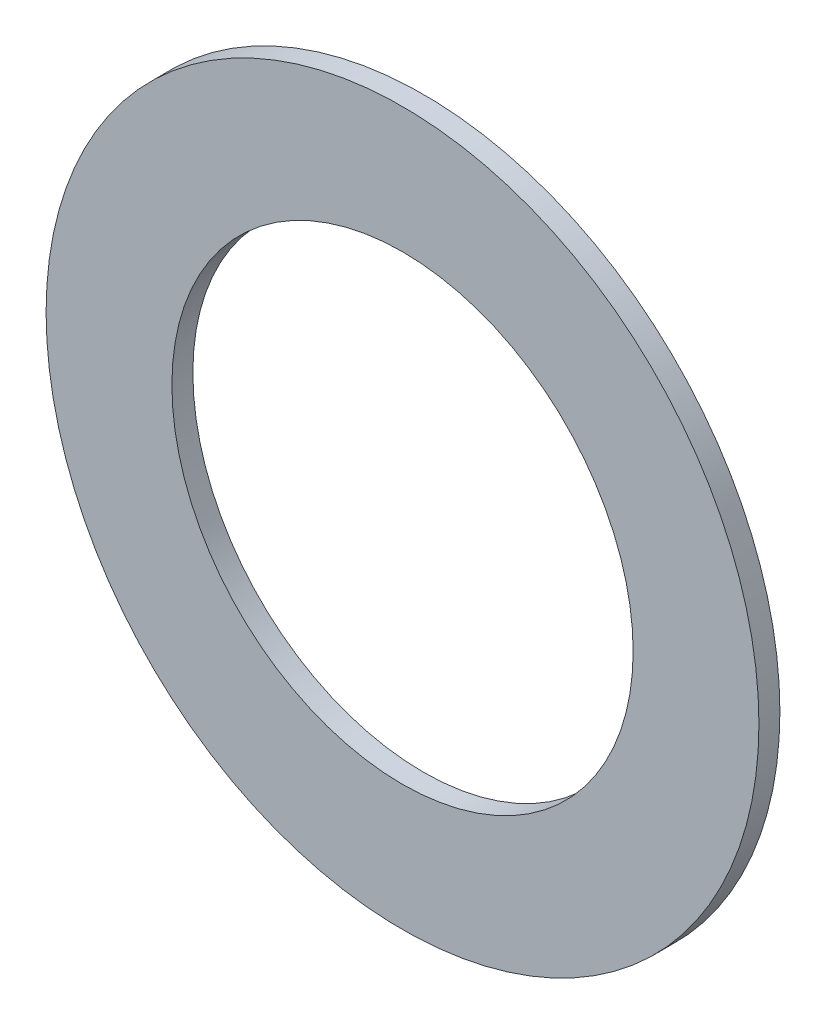
SolidWorks part; units mm, degrees
ref_plane "Front Plane" through (0, 0, 0) normal (0, 0, 1) x (1, 0, 0)
ref_plane "Top Plane" through (0, 0, 0) normal (0, 1, 0) x (1, 0, 0)
ref_plane "Right Plane" through (0, 0, 0) normal (1, 0, 0) x (0, 0, -1)
other "Configuration Table"
sketch "Sketch1" plane through (0, 0, 0) normal (0, 0, 1) x (1, 0, 0)
  circle A0 centre (0, 0) radius 5.5 construction
  circle A1 centre (0, 0) radius 8.5
  circle A2 centre (0, 0) radius 8.5
  circle A3 centre (0, 0) radius 5.5
  dimension "D1" = 0
extrude "Boss-Extrude1" add sketch "Sketch1" along normal blind 0.5
